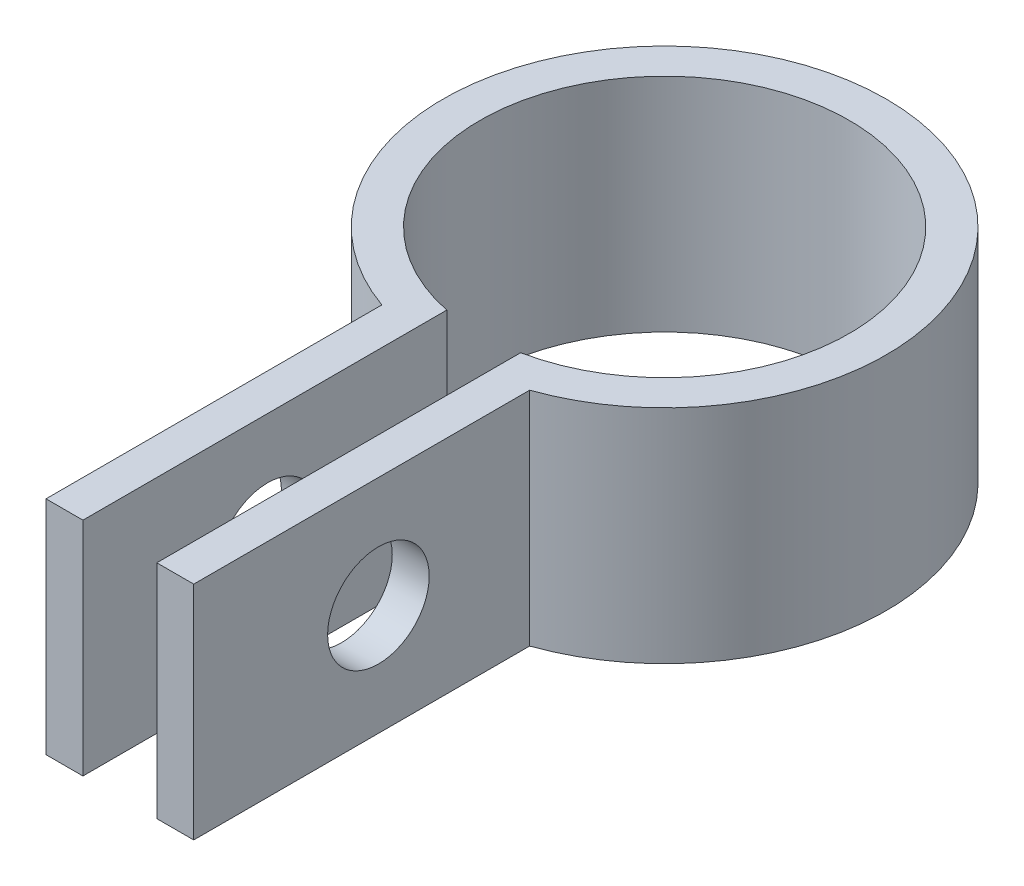
from build123d import *

# Parameters (mm, degrees)
EXTRUDE_1_DEPTH          = 12
CUT_EXTRUDE_1_DEPTH      = 65.815121692
CUT_EXTRUDE_1_DEPTH_BACK = 65.815121692
SKETCH_2_R               = 5.5


with BuildPart() as part:
    # 草图1 → 凸台-拉伸1 (new, symmetric)
    with BuildSketch(Plane(origin=(0, 0, 0), x_dir=(1, 0, 0), z_dir=(0, 1, 0))):
        with BuildLine():
            Line((8, -59), (4, -59))
            Line((4, -59), (4, -19.595917942))
            ThreePointArc((4, -19.595917942), (0, 20), (-4, -19.595917942))
            Line((-4, -19.595917942), (-4, -59))
            Line((-4, -59), (-8, -59))
            Line((-8, -59), (-8, -22.627416998))
            ThreePointArc((-8, -22.627416998), (0, 24), (8, -22.627416998))
            Line((8, -22.627416998), (8, -59))
        make_face()
    extrude(amount=EXTRUDE_1_DEPTH, both=True)

    # 草图2 → 切除-拉伸1 (cut, two sides: drawn at the far end of the back side and taken through both)
    with BuildSketch(Plane(origin=(0, 0, 0), x_dir=(0, 0, -1), z_dir=(1, 0, 0)).offset(-CUT_EXTRUDE_1_DEPTH_BACK)):
        with Locations((-39, 0)):
            Circle(SKETCH_2_R)
    extrude(amount=CUT_EXTRUDE_1_DEPTH + CUT_EXTRUDE_1_DEPTH_BACK, mode=Mode.SUBTRACT)


solid = part.part
